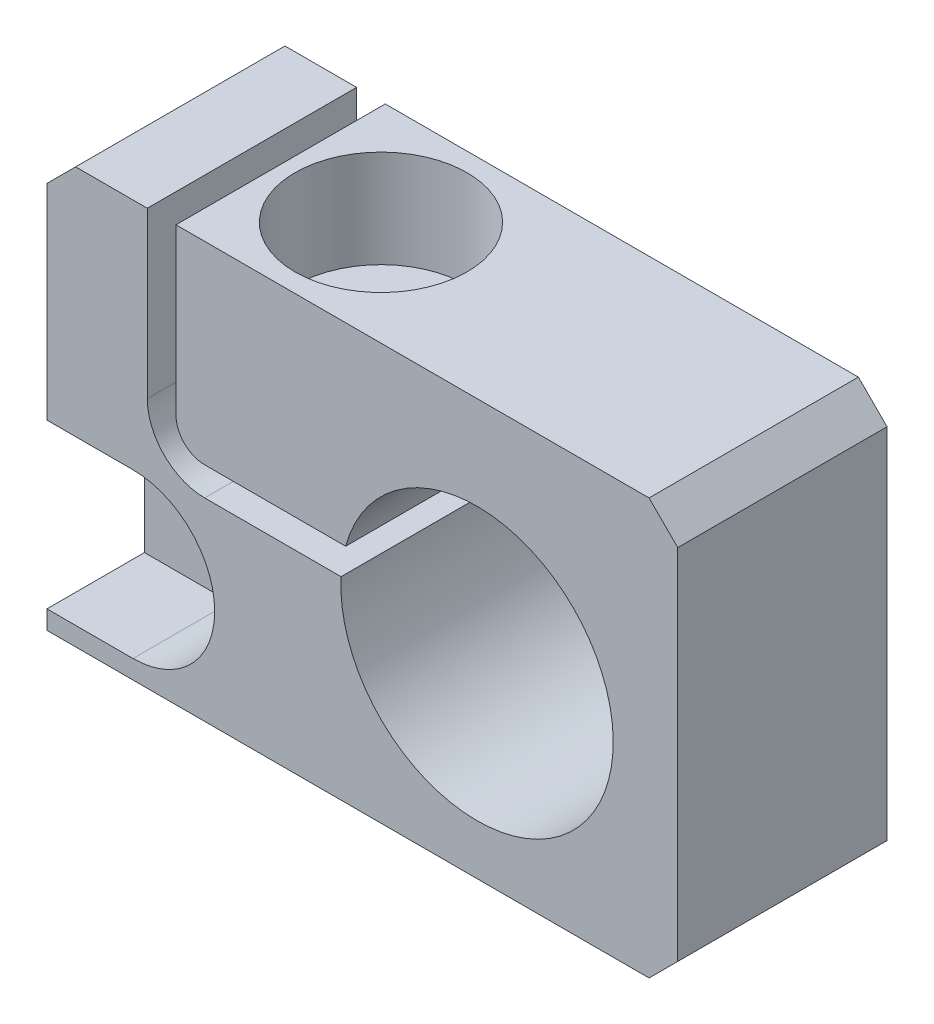
from build123d import *

# Parameters (mm, degrees)
SKETCH1_W                                            = 22
SKETCH1_H                                            = 14.5
BOSS_EXTRUDE1_DEPTH                                  = 7.3
SKETCH2_R                                            = 4.75
CUT_EXTRUDE1_DEPTH                                   = 16.061623418
F_3_4_3_4_DIAMETER_HOLE1_D                           = 3.4
SKETCH5_W                                            = 15
SKETCH5_H                                            = 1
CUT_EXTRUDE2_DEPTH                                   = 16.061623418
SKETCH6_W                                            = 1
SKETCH6_H                                            = 6.75
CUT_EXTRUDE3_DEPTH                                   = 17
FILLET1_R                                            = 2
FILLET2_R                                            = 1
SKETCH7_W                                            = 1.25
SKETCH7_H                                            = 6.75
HOLE_SIZE_PER_SOCKET_HEAD_CAP_SCREW_TYPE_D           = 3.4
HOLE_SIZE_PER_SOCKET_HEAD_CAP_SCREW_TYPE_DEPTH       = 7.749
HOLE_SIZE_PER_SOCKET_HEAD_CAP_SCREW_TYPE_CBORE_D     = 6
HOLE_SIZE_PER_SOCKET_HEAD_CAP_SCREW_TYPE_CBORE_DEPTH = 3.4
CUT_EXTRUDE4_DEPTH                                   = 3.4
CHAMFER1_SIZE                                        = 1


with BuildPart() as part:
    # Sketch1 → Boss-Extrude1 (new body)
    with BuildSketch(Plane.XY):
        Rectangle(SKETCH1_W, SKETCH1_H)
    extrude(amount=BOSS_EXTRUDE1_DEPTH)

    # Sketch2 → Cut-Extrude1 (cut, through all)
    with BuildSketch(Plane.XY.offset(7.3)):
        with Locations((4, -0.75)):
            Circle(SKETCH2_R)
    extrude(amount=-CUT_EXTRUDE1_DEPTH, mode=Mode.SUBTRACT)

    # Ø3.4 (3.4) Diameter Hole1 (through all)
    with Locations(Plane.XY.offset(7.3)):
        with Locations((-8, -3.75)):
            Hole(F_3_4_3_4_DIAMETER_HOLE1_D / 2)

    # Sketch5 → Cut-Extrude2 (cut, through all)
    with BuildSketch(Plane.XY.offset(7.3)):
        Rectangle(SKETCH5_W, SKETCH5_H)
    extrude(amount=-CUT_EXTRUDE2_DEPTH, mode=Mode.SUBTRACT)

    # Sketch6 → Cut-Extrude3 (cut)
    with BuildSketch(Plane.XY.offset(7.3)):
        with Locations((-7, 3.875)):
            Rectangle(SKETCH6_W, SKETCH6_H)
    extrude(amount=-CUT_EXTRUDE3_DEPTH, mode=Mode.SUBTRACT)

    # Fillet1
    fillet1_edges = [part.edges().sort_by_distance(p)[0] for p in [
        (-7.5, -0.5, 3.65),
    ]]
    fillet(fillet1_edges, radius=FILLET1_R)

    # Fillet2
    fillet2_edges = [part.edges().sort_by_distance(p)[0] for p in [
        (-6.5, 0.5, 3.65),
    ]]
    fillet(fillet2_edges, radius=FILLET2_R)

    # Sketch7 → M3 Tapped Hole1 (revolve, cut)
    with BuildSketch(Plane(origin=(-3, -0.5, 3.65), x_dir=(0, 0, 1), z_dir=(1, 0, 0))):
        with Locations((0.625, 3.375)):
            Rectangle(SKETCH7_W, SKETCH7_H)
    revolve(axis=Axis((-3, 5.85, 3.65), (0, -1, 0)), mode=Mode.SUBTRACT)

    # Hole size per socket head cap screw type 3
    with Locations(Plane(origin=(0, 7.25, 0), x_dir=(1, 0, 0), z_dir=(0, 1, 0))):
        with Locations((-3, -3.65)):
            CounterBoreHole(HOLE_SIZE_PER_SOCKET_HEAD_CAP_SCREW_TYPE_D / 2, HOLE_SIZE_PER_SOCKET_HEAD_CAP_SCREW_TYPE_CBORE_D / 2, HOLE_SIZE_PER_SOCKET_HEAD_CAP_SCREW_TYPE_CBORE_DEPTH, depth=HOLE_SIZE_PER_SOCKET_HEAD_CAP_SCREW_TYPE_DEPTH)

    # Sketch13 → Cut-Extrude4 (cut)
    with BuildSketch(Plane.XY.offset(7.3)):
        with BuildLine():
            Line((-8, -6.6), (-13.475777531, -6.6))
            ThreePointArc((-13.475777531, -6.6), (-16.325777531, -3.75), (-13.475777531, -0.9))
            Line((-13.475777531, -0.9), (-8, -0.9))
            ThreePointArc((-8, -0.9), (-5.15, -3.75), (-8, -6.6))
        make_face()
    extrude(amount=-CUT_EXTRUDE4_DEPTH, mode=Mode.SUBTRACT)

    # Chamfer1
    chamfer1_edges = [part.edges().sort_by_distance(p)[0] for p in [
        (11, -7.25, 3.65),
        (-11, 7.25, 3.65),
        (11, 7.25, 3.65),
    ]]
    chamfer(chamfer1_edges, length=CHAMFER1_SIZE)


solid = part.part
